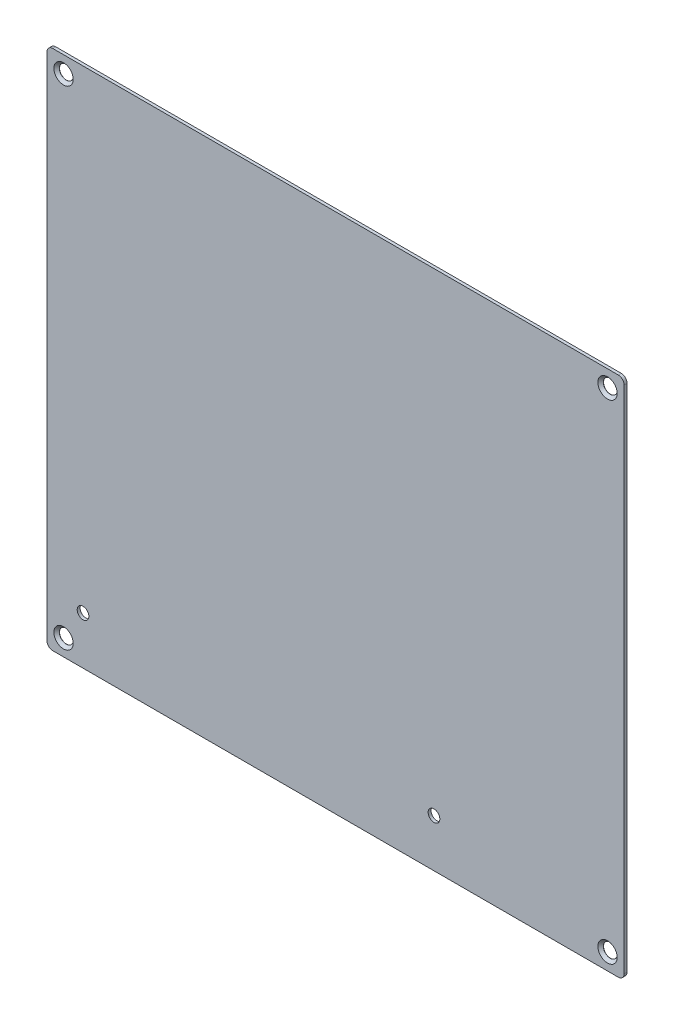
from build123d import *

# Parameters (mm, degrees)
SKETCH_1_W                       = 296
SKETCH_1_H                       = 267.5
EXTRUDE_1_DEPTH                  = 1.5
HOLE_WIZARD_7_1_7_1_2_AT_2_COUNT = 2
HOLE_WIZARD_7_1_7_1_2_AT_2_PITCH = 250.5
HOLE_WIZARD_7_1_7_1_2_AT_3_COUNT = 2
HOLE_WIZARD_7_1_7_1_2_AT_3_PITCH = 374.9549973
HOLE_WIZARD_7_1_7_1_2_AT_4_COUNT = 2
HOLE_WIZARD_7_1_7_1_2_AT_4_PITCH = 279
FILLET_1_R                       = 3
SKETCH_6_R                       = 3
CUT_EXTRUDE_1_DEPTH              = 1.5


with BuildPart() as part:
    # 草图1 → 凸台-拉伸1 (new body)
    with BuildSketch(Plane.XY):
        with Locations((-237.5, 200.75)):
            Rectangle(SKETCH_1_W, SKETCH_1_H)
    extrude(amount=-EXTRUDE_1_DEPTH)

    # 草图4 → Ø7.1 (7.1) 直径孔2 (revolve, cut)
    with BuildSketch(Plane(origin=(-377, 326, 0), x_dir=(0, -1, 0), z_dir=(1, 0, 0))):
        Polygon((0, 0), (0, 1.5), (3.55, 1.5), (3.55, 1.4), (4.95, 0), align=None)
    hole_wizard_7_1_7_1_2 = revolve(axis=Axis((-377, 326, 6.35), (0, 0, -1)), mode=Mode.SUBTRACT)

    # Ø7.1 (7.1) 直径孔2 at 2: Ø7.1 (7.1) 直径孔2 ×2
    with Locations(*[(0, -i * HOLE_WIZARD_7_1_7_1_2_AT_2_PITCH, 0) for i in range(1, HOLE_WIZARD_7_1_7_1_2_AT_2_COUNT)]):
        add(hole_wizard_7_1_7_1_2, mode=Mode.SUBTRACT)

    # Ø7.1 (7.1) 直径孔2 at 3: Ø7.1 (7.1) 直径孔2 ×2
    with Locations(*[Vector(0.7440892960736261, -0.6680801744316739, 0) * (i * HOLE_WIZARD_7_1_7_1_2_AT_3_PITCH) for i in range(1, HOLE_WIZARD_7_1_7_1_2_AT_3_COUNT)]):
        add(hole_wizard_7_1_7_1_2, mode=Mode.SUBTRACT)

    # Ø7.1 (7.1) 直径孔2 at 4: Ø7.1 (7.1) 直径孔2 ×2
    with Locations(*[(i * HOLE_WIZARD_7_1_7_1_2_AT_4_PITCH, 0, 0) for i in range(1, HOLE_WIZARD_7_1_7_1_2_AT_4_COUNT)]):
        add(hole_wizard_7_1_7_1_2, mode=Mode.SUBTRACT)

    # 圆角1
    fillet_1_edges = [part.edges().sort_by_distance(p)[0] for p in [
        (-385.5, 67, -0.75),
        (-385.5, 334.5, -0.75),
        (-89.5, 334.5, -0.75),
        (-89.5, 67, -0.75),
    ]]
    fillet(fillet_1_edges, radius=FILLET_1_R)

    # 草图6 → 切除-拉伸1 (cut)
    with BuildSketch(Plane.XY):
        with Locations((-367, 91.5)):
            Circle(SKETCH_6_R)
        with Locations((-187, 91.5)):
            Circle(SKETCH_6_R)
    extrude(amount=-CUT_EXTRUDE_1_DEPTH, mode=Mode.SUBTRACT)


solid = part.part
